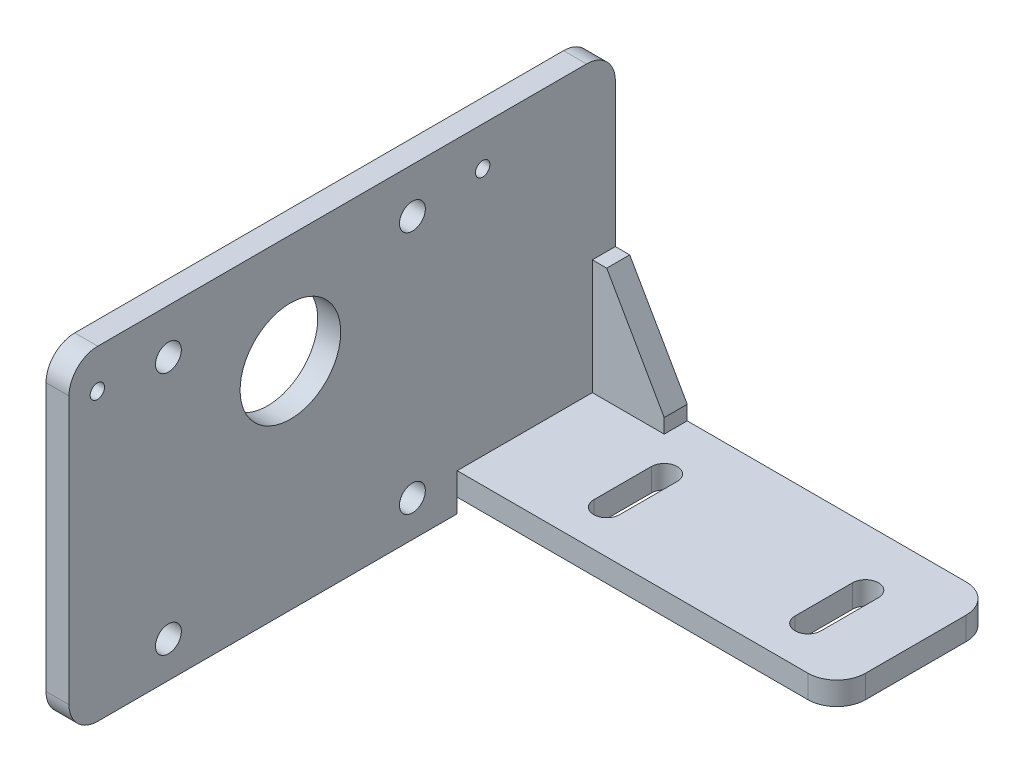
SolidWorks part; units mm, degrees
ref_plane "前视基准面" through (0, 0, 0) normal (0, 0, 1) x (1, 0, 0)
ref_plane "上视基准面" through (0, 0, 0) normal (0, 1, 0) x (1, 0, 0)
ref_plane "右视基准面" through (0, 0, 0) normal (1, 0, 0) x (0, 0, -1)
sketch "草图1" plane through (0, 0, 0) normal (0, 0, 1) x (1, 0, 0)
  line L0 (0, 108) -> (0, 0)
  line L1 (0, 0) -> (140, 0)
  dimension "D1" = 140
  dimension "D2" = 108
extrude "拉伸-薄壁1" add sketch "草图1" against normal mid plane 190 thin thin type one direction reverse wall 8
sketch "草图2" plane through (0, 8, 0) normal (0, 1, 0) x (1, 0, 0)
  line L0 (140, 0) -> (80, 0) construction
  line L1 (140, 95) -> (140, -95) construction
  line L3 (115, -65) -> (45, -65) construction
  line L4 (115, -65) -> (115, 65) construction
  line L5 (115, 65) -> (45, 65) construction
  line L6 (45, -65) -> (45, 65) construction
  line L7 (115, -65) -> (45, 65) construction
  line L8 (115, 65) -> (45, -65) construction
  circle A0 centre (115, 65) radius 4.5
  circle A1 centre (45, 65) radius 4.5
  circle A2 centre (115, -65) radius 4.5
  circle A3 centre (45, -65) radius 4.5
  dimension "D4" = 9
  dimension "D1" = 70
  dimension "D2" = 25
  dimension "D3" = 130
extrude "切除-拉伸1" cut sketch "草图2" against normal blind 10
sketch "草图4" plane through (0, 0, 95) normal (0, 0, 1) x (1, 0, 0)
  line L0 (8, 48) -> (13, 48)
  line L1 (8, 108) -> (8, 8) construction
  line L2 (13, 48) -> (33, 13)
  line L3 (33, 13) -> (33, 8)
  line L4 (8, 8) -> (140, 8) construction
  line L5 (33, 8) -> (8, 8)
  line L6 (8, 8) -> (8, 48)
  dimension "D1" = 5
  dimension "D2" = 25
  dimension "D3" = 40
extrude "凸台-拉伸1" add sketch "草图4" against normal blind 8 separate body
sketch "草图5" plane through (8, 0, 0) normal (1, 0, 0) x (0, 0, -1)
  line L0 (-18, 105) -> (-18, 50) construction
  line L2 (95, 0) -> (-95, 0) construction
  line L3 (-60.4264, 92.4264) -> (24.4264, 92.4264) construction
  line L4 (-60.4264, 92.4264) -> (-60.4264, 7.5736) construction
  line L5 (-60.4264, 7.5736) -> (24.4264, 7.5736) construction
  line L6 (24.4264, 92.4264) -> (24.4264, 7.5736) construction
  line L7 (-60.4264, 92.4264) -> (24.4264, 7.5736) construction
  line L8 (-60.4264, 7.5736) -> (24.4264, 92.4264) construction
  line L9 (-95, 108) -> (-95, 8) construction
  circle A0 centre (-60.4264, 92.4264) radius 4.5
  circle A1 centre (-60.4264, 7.5736) radius 4.5
  circle A2 centre (24.4264, 7.5736) radius 4.5
  circle A3 centre (24.4264, 92.4264) radius 4.5
  circle A5 centre (-18, 50) radius 60 construction
  circle A6 centre (-18, 70) radius 17.5
  dimension "D4" = 9
  dimension "D7" = 120
  dimension "D2" = 35
  dimension "D3" = 20
  dimension "D1" = 70
  dimension "D6" = 77
extrude "切除-拉伸2" cut sketch "草图5" against normal through all
fillet "圆角1" radius 10 4 edges at (140, 4, 95) (140, 4, -95) (4, 108, -95) (4, 108, 95)
mirror "镜向2" about plane through (0, 0, 0) normal (0, 0, 1) of bodies 103
sketch "草图7" plane through (0, 8, 0) normal (0, 1, 0) x (1, 0, 0)
  line L0 (45, 55) -> (45, 75) construction
  line L1 (40.5, 55) -> (40.5, 75)
  line L2 (49.5, 55) -> (49.5, 75)
  line L3 (115, 55) -> (115, 75) construction
  line L4 (110.5, 55) -> (110.5, 75)
  line L5 (119.5, 55) -> (119.5, 75)
  line L6 (115, -75) -> (115, -55) construction
  line L7 (110.5, -75) -> (110.5, -55)
  line L8 (119.5, -75) -> (119.5, -55)
  line L9 (45, -75) -> (45, -55) construction
  line L10 (40.5, -75) -> (40.5, -55)
  line L11 (49.5, -75) -> (49.5, -55)
  arc A0 (40.5, 55) -> (49.5, 55) centre (45, 55) ccw
  arc A1 (49.5, 75) -> (40.5, 75) centre (45, 75) ccw
  arc A2 (110.5, 55) -> (119.5, 55) centre (115, 55) ccw
  arc A3 (119.5, 75) -> (110.5, 75) centre (115, 75) ccw
  arc A4 (110.5, -75) -> (119.5, -75) centre (115, -75) ccw
  arc A5 (119.5, -55) -> (110.5, -55) centre (115, -55) ccw
  arc A6 (40.5, -75) -> (49.5, -75) centre (45, -75) ccw
  arc A7 (49.5, -55) -> (40.5, -55) centre (45, -55) ccw
  point P2 (45, 65)
  point P9 (115, 65)
  point P17 (115, -65)
  point P25 (45, -65)
  dimension "D1" = 9
  dimension "D2" = 20
extrude "切除-拉伸4" cut sketch "草图7" against normal blind 10
sketch "草图8" plane through (0, 8, 0) normal (0, 1, 0) x (1, 0, 0)
  line L0 (140, 85) -> (140, -85) construction
  line L1 (140, 40) -> (8, 40)
  line L2 (140, 40) -> (140, -123.8203)
  line L3 (140, -123.8203) -> (8, -123.8203)
  line L4 (8, 40) -> (8, -123.8203)
  line L8 (8, 95) -> (130, 95) construction
  line L9 (8, 19.9467) -> (8, -55.9467) construction
  dimension "D1" = 55
extrude "切除-拉伸5" cut sketch "草图8" against normal blind 10
fillet "圆角2" radius 10 1 edges at (140, 4, -40)
delete or keep bodies "实体-删除/保留 1" type delete bodies bodies 103
sketch "草图9" plane through (0, 0, 0) normal (0, -1, 0) x (1, 0, 0)
  line L1 (8, -40) -> (0, -40)
  line L2 (8, -40) -> (8, 95)
  line L3 (8, 95) -> (0, 95)
  line L4 (0, -40) -> (0, 95)
extrude "凸台-拉伸2" add sketch "草图9" along normal blind 5
fillet "圆角3" radius 10 1 edges at (4, -5, 95)
sketch "草图10" plane through (8, 0, 0) normal (1, 0, 0) x (0, 0, -1)
  circle A0 centre (-85.1423, 94.5) radius 2.5
  circle A1 centre (48.8577, 94.5) radius 2.5
  dimension "D1" = 5
extrude "切除-拉伸6" cut sketch "草图10" against normal blind 10
